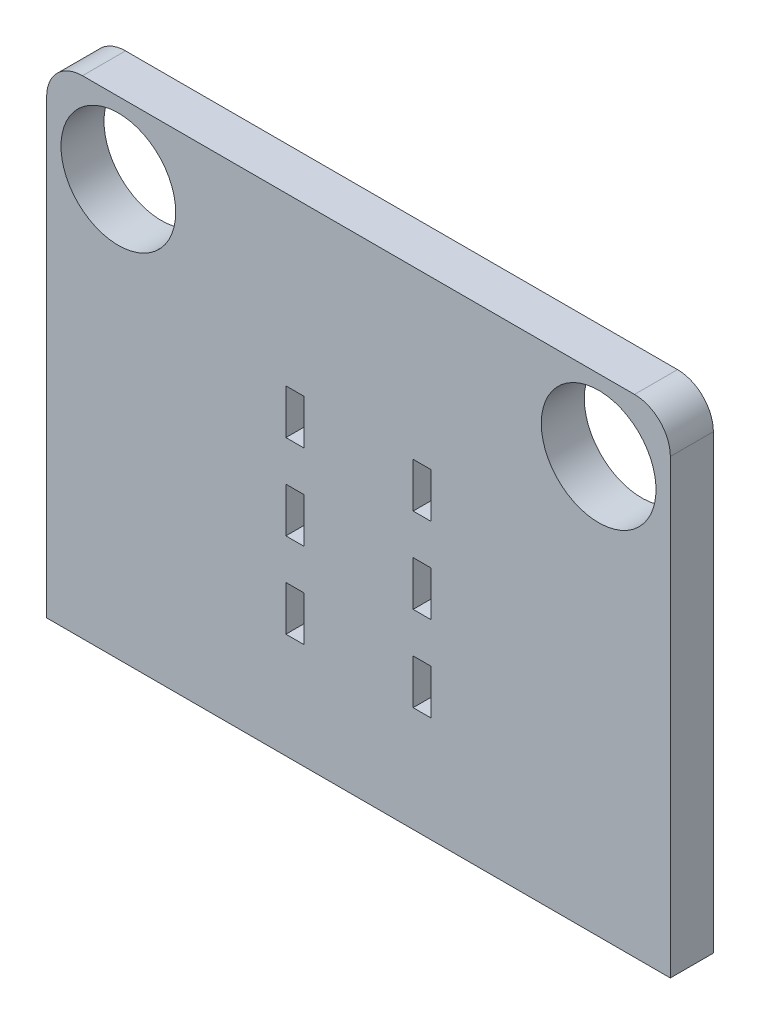
from build123d import *

# Parameters (mm, degrees)
SKETCH_1_W      = 174
SKETCH_1_H      = 136
SKETCH_1_R      = 16
SKETCH_1_W_2    = 5
SKETCH_1_H_2    = 12.5
EXTRUDE_1_DEPTH = 12
FILLET_2_R      = 10


with BuildPart() as part:
    # 草图1 → 凸台-拉伸1 (new body)
    with BuildSketch(Plane.XY):
        with Locations((-22.664999192, 1.659931171)):
            Rectangle(SKETCH_1_W, SKETCH_1_H)
        with Locations((-89.664999192, 49.659931171)):
            Circle(SKETCH_1_R, mode=Mode.SUBTRACT)
        with Locations(Location((44.335000808, 49.659931171, 0), (0, 0, 180))):
            Circle(SKETCH_1_R, mode=Mode.SUBTRACT)
        with Locations((-40.414999192, 16.852464835)):
            Rectangle(SKETCH_1_W_2, SKETCH_1_H_2, mode=Mode.SUBTRACT)
        with Locations((-40.414999192, -6.897535165)):
            Rectangle(SKETCH_1_W_2, SKETCH_1_H_2, mode=Mode.SUBTRACT)
        with Locations((-40.414999192, -30.647535165)):
            Rectangle(SKETCH_1_W_2, SKETCH_1_H_2, mode=Mode.SUBTRACT)
        with Locations((-4.914999192, -30.647535165)):
            Rectangle(SKETCH_1_W_2, SKETCH_1_H_2, mode=Mode.SUBTRACT)
        with Locations((-4.914999192, -6.897535165)):
            Rectangle(SKETCH_1_W_2, SKETCH_1_H_2, mode=Mode.SUBTRACT)
        with Locations((-4.914999192, 16.852464835)):
            Rectangle(SKETCH_1_W_2, SKETCH_1_H_2, mode=Mode.SUBTRACT)
    extrude(amount=EXTRUDE_1_DEPTH)

    # 圆角2
    fillet_2_edges = [part.edges().sort_by_distance(p)[0] for p in [
        (64.335000808, 69.659931171, 6),
        (-109.664999192, 69.659931171, 6),
    ]]
    fillet(fillet_2_edges, radius=FILLET_2_R)


solid = part.part
